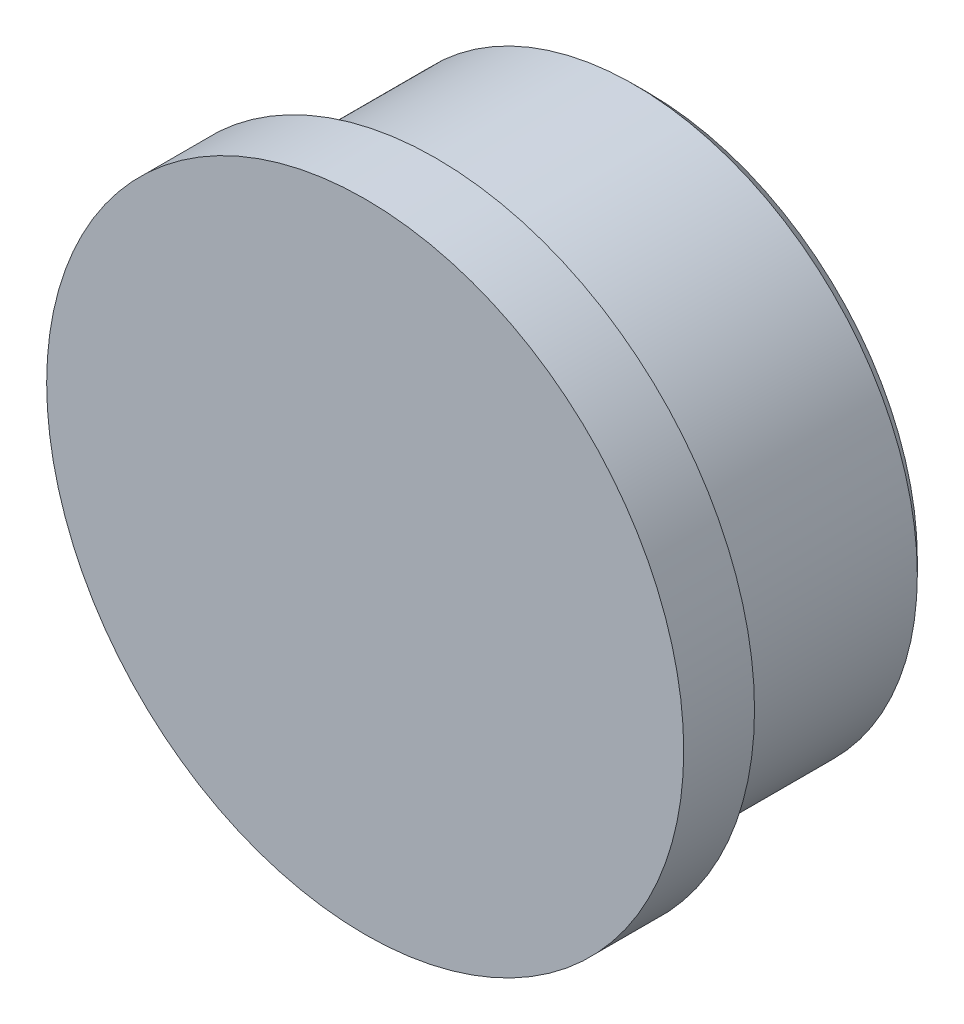
from build123d import *

# Parameters (mm, degrees)
SKETCH_1_R      = 40
EXTRUDE_1_DEPTH = 30
SKETCH_2_R      = 45
EXTRUDE_2_DEPTH = 10
CHAMFER_1_SIZE  = 2


with BuildPart() as part:
    # 草图1 → 凸台-拉伸1 (new body)
    with BuildSketch(Plane.XY):
        Circle(SKETCH_1_R)
    extrude(amount=EXTRUDE_1_DEPTH)

    # 草图2 → 凸台-拉伸2 (add)
    with BuildSketch(Plane.XY.offset(30)):
        Circle(SKETCH_2_R)
    extrude(amount=EXTRUDE_2_DEPTH)

    # 倒角1
    chamfer_1_edges = [part.edges().sort_by_distance(p)[0] for p in [
        (-40, 0, 0),
    ]]
    chamfer(chamfer_1_edges, length=CHAMFER_1_SIZE)


solid = part.part
